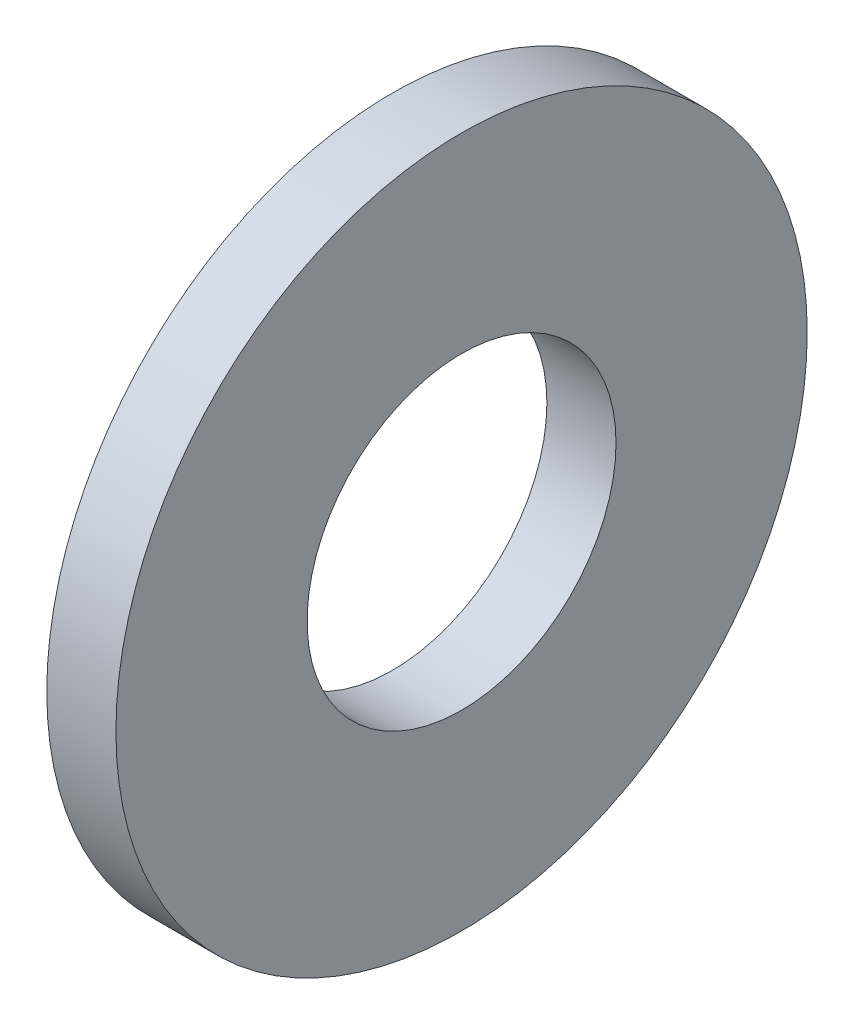
SolidWorks part; units mm, degrees
ref_plane "Plane1" through (0, 0, 0) normal (0, 0, 1) x (1, 0, 0)
ref_plane "Plane2" through (0, 0, 0) normal (0, 1, 0) x (1, 0, 0)
ref_plane "Plane3" through (0, 0, 0) normal (1, 0, 0) x (0, 0, -1)
other "Configuration Table"
sketch "Sketch1" plane through (0, 0, 0) normal (1, 0, 0) x (0, 0, -1)
  circle A0 centre (0, 0) radius 3.575
  circle A1 centre (0, 0) radius 8
  dimension "Insid_dia" = 7.15
  dimension "OutsideDia" = 16
extrude "Base-Extrude" add sketch "Sketch1" along normal blind 1.6
